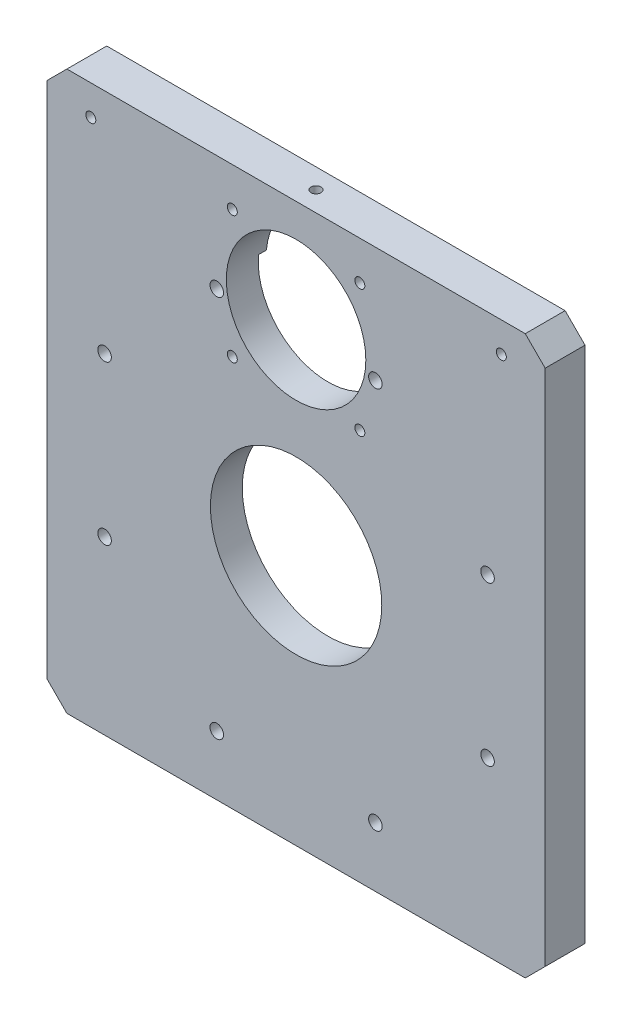
SolidWorks part; units mm, degrees
material "Q235A"
ref_plane "前视基准面" through (0, 0, 0) normal (0, 0, 1) x (1, 0, 0)
ref_plane "上视基准面" through (0, 0, 0) normal (0, 1, 0) x (1, 0, 0)
ref_plane "右视基准面" through (0, 0, 0) normal (1, 0, 0) x (0, 0, -1)
sketch "草图1" plane through (0, 0, 0) normal (0, 0, 1) x (1, 0, 0)
  line L1 (-125, -140) -> (125, -140)
  line L2 (-125, -140) -> (-125, 140)
  line L3 (-125, 140) -> (125, 140)
  line L4 (125, -140) -> (125, 140)
  line L5 (-125, -140) -> (125, 140) construction
  line L6 (-125, 140) -> (125, -140) construction
  circle A0 centre (0, -14) radius 43
  circle A1 centre (0, 88.5) radius 35
  point P0 (0, 0)
  dimension "D3" = 86
  dimension "D5" = 70
  dimension "D6" = 102.5
  dimension "D1" = 280
  dimension "D2" = 250
  dimension "D4" = 126
extrude "凸台-拉伸1" add sketch "草图1" along normal blind 20
hole_wizard "M8 螺纹孔1" positions "草图2" profile "草图3" tap size "M8" standard "ISO" end condition through all
sketch "草图2" plane through (0, 0, 20) normal (0, 0, 1) x (1, 0, 0)
  line L1 (0, -14) -> (-39.7991, 82.0835) construction
  line L2 (0, -14) -> (0, 140) construction
  line L3 (125, 140) -> (-125, 140) construction
  point P0 (-39.7991, 82.0835)
  point P12 (39.7991, 82.0835)
  point P13 (96.0835, 25.7991)
  point P14 (96.0835, -53.7991)
  point P15 (39.7991, -110.0835)
  point P16 (-39.7991, -110.0835)
  point P17 (-96.0835, -53.7991)
  point P18 (-96.0835, 25.7991)
  dimension "D3" = 104
  dimension "D2" = 8
sketch "草图3" plane through (-39.7991, 82.0835, 20) normal (1, 0, 0) x (0, -1, 0)
  line L0 (0, 0) -> (0, 20)
  line L1 (0, 20) -> (3.4, 20)
  line L2 (3.4, 20) -> (3.4, 0)
  line L5 (3.4, 0) -> (0, 0)
  line L11 (0, -6.35) -> (0, 107.95) construction
  dimension "通孔螺纹孔钻头直径" = 6.8
  dimension "通孔螺纹孔钻头深度" = 20
cosmetic thread "孔螺蚊线1" parameters "D2"=8
cosmetic thread "孔螺蚊线2" parameters "D2"=8
cosmetic thread "孔螺蚊线3" parameters "D2"=8
cosmetic thread "孔螺蚊线4" parameters "D2"=8
cosmetic thread "孔螺蚊线5" parameters "D2"=8
cosmetic thread "孔螺蚊线6" parameters "D2"=8
cosmetic thread "孔螺蚊线7" parameters "D2"=8
cosmetic thread "孔螺蚊线12" parameters "D2"=8
hole_wizard "M6 螺纹孔1" positions "草图4" profile "草图5" tap size "M6" standard "ISO" end condition through all
sketch "草图4" plane through (0, 0, 0) normal (0, 0, -1) x (-1, 0, 0)
  line L1 (-32, 56.5) -> (32, 56.5)
  line L2 (-32, 56.5) -> (-32, 120.5)
  line L3 (-32, 120.5) -> (32, 120.5)
  line L4 (32, 56.5) -> (32, 120.5)
  line L5 (-32, 56.5) -> (32, 120.5) construction
  line L6 (-32, 120.5) -> (32, 56.5) construction
  point P1 (0, 88.5)
  point P2 (32, 120.5)
  point P5 (-32, 56.5)
  point P6 (-32, 120.5)
  point P7 (32, 56.5)
  dimension "D1" = 64
  dimension "D2" = 64
sketch "草图5" plane through (0, 88.5, 0) normal (1, 0, 0) x (0, 1, 0)
  line L0 (0, 0) -> (0, 20)
  line L1 (0, 20) -> (2.5, 20)
  line L2 (2.5, 20) -> (2.5, 0)
  line L5 (2.5, 0) -> (0, 0)
  line L11 (0, -6.35) -> (0, 107.95) construction
  dimension "通孔螺纹孔钻头直径" = 5
  dimension "通孔螺纹孔钻头深度" = 20
cosmetic thread "孔螺蚊线8" parameters "D2"=6
cosmetic thread "孔螺蚊线9" parameters "D2"=6
cosmetic thread "孔螺蚊线10" parameters "D2"=6
cosmetic thread "孔螺蚊线11" parameters "D2"=6
sketch "草图6" plane through (0, 0, 0) normal (0, 0, -1) x (-1, 0, 0)
  circle A0 centre (0, -14) radius 111
  dimension "D1" = 222
extrude "切除-拉伸1" cut sketch "草图6" against normal blind 4
chamfer "倒角1" distance 10 angle 45 4 edges at (-125, -140, 10) (125, -140, 10) (125, 140, 10) (-125, 140, 10)
hole_wizard "M6 螺纹孔2" positions "草图7" profile "草图8" tap size "M6" standard "ISO" end condition through all
sketch "草图7" plane through (0, 0, 0) normal (0, 0, -1) x (-1, 0, 0)
  line L0 (0, 0) -> (0, 140) construction
  line L1 (-115, 140) -> (115, 140) construction
  point P0 (103, 125)
  point P2 (-103, 125)
  dimension "D1" = 15
  dimension "D2" = 206
sketch "草图8" plane through (-103, 125, 0) normal (1, 0, 0) x (0, 1, 0)
  line L0 (0, 0) -> (0, 20)
  line L1 (0, 20) -> (2.5, 20)
  line L2 (2.5, 20) -> (2.5, 0)
  line L5 (2.5, 0) -> (0, 0)
  line L11 (0, -6.35) -> (0, 107.95) construction
  dimension "通孔螺纹孔钻头直径" = 5
  dimension "通孔螺纹孔钻头深度" = 20
cosmetic thread "孔螺蚊线13" parameters "D2"=6
cosmetic thread "孔螺蚊线14" parameters "D2"=6
hole_wizard "M6 螺纹孔3" positions "草图9" profile "草图10" tap size "M6" standard "ISO"
sketch "草图9" plane through (0, 140, 0) normal (0, 1, 0) x (1, 0, 0)
  line L0 (0, 0) -> (0, -20)
  line L1 (115, -20) -> (-115, -20) construction
  point P0 (0, -10)
sketch "草图10" plane through (0, 140, 10) normal (1, 0, 0) x (0, 0, 1)
  line L0 (0, 0) -> (0, 16.5022)
  line L1 (0, 16.5022) -> (2.5, 15)
  line L2 (2.5, 15) -> (2.5, 0)
  line L5 (2.5, 0) -> (0, 0)
  line L10 (0, 16.5022) -> (-2.5, 15) construction
  line L11 (0, -6.35) -> (0, 107.95) construction
  dimension "螺纹孔钻头直径" = 5
  dimension "螺纹孔钻头深度" = 15
  dimension "导头角度" = 118
cosmetic thread "孔螺蚊线15" parameters "D1"=12, "D2"=6
